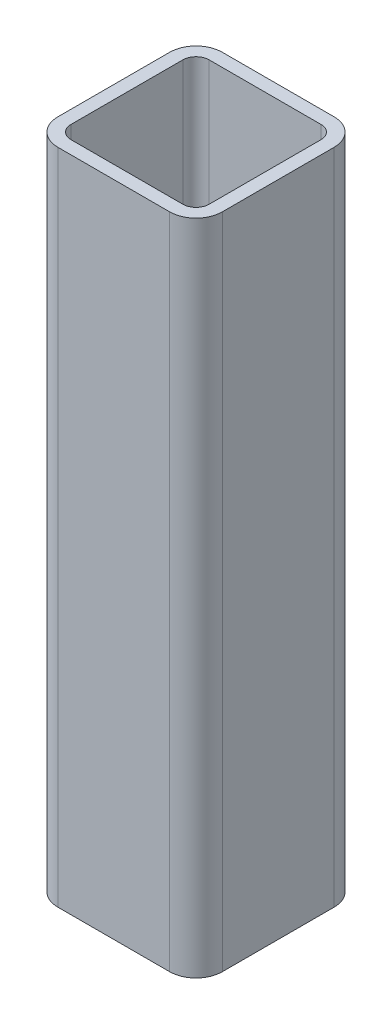
from build123d import *

# Parameters (mm, degrees)
GB_T_6728_2002_SQUARE_HOLLOW_SECTION_STE_DEPTH = 100


with BuildPart() as part:
    # Sketch14 → Gb／t 6728—2002 Square hollow section steel 25×2-example.com(1) (new body)
    with BuildSketch(Plane(origin=(0, 0, 0), x_dir=(-1, 0, 0), z_dir=(0, 1, 0))):
        with BuildLine():
            Line((-8.5, -12.5), (8.5, -12.5))
            ThreePointArc((8.5, -12.5), (11.328427125, -11.328427125), (12.5, -8.5))
            Line((12.5, -8.5), (12.5, 8.5))
            ThreePointArc((12.5, 8.5), (11.328427125, 11.328427125), (8.5, 12.5))
            Line((8.5, 12.5), (-8.5, 12.5))
            ThreePointArc((-8.5, 12.5), (-11.328427125, 11.328427125), (-12.5, 8.5))
            Line((-12.5, 8.5), (-12.5, -8.5))
            ThreePointArc((-12.5, -8.5), (-11.328427125, -11.328427125), (-8.5, -12.5))
        make_face()
        with BuildLine():
            Line((-8.5, -10.5), (8.5, -10.5))
            ThreePointArc((8.5, -10.5), (9.914213562, -9.914213562), (10.5, -8.5))
            Line((10.5, -8.5), (10.5, 8.5))
            ThreePointArc((10.5, 8.5), (9.914213562, 9.914213562), (8.5, 10.5))
            Line((8.5, 10.5), (-8.5, 10.5))
            ThreePointArc((-8.5, 10.5), (-9.914213562, 9.914213562), (-10.5, 8.5))
            Line((-10.5, 8.5), (-10.5, -8.5))
            ThreePointArc((-10.5, -8.5), (-9.914213562, -9.914213562), (-8.5, -10.5))
        make_face(mode=Mode.SUBTRACT)
    extrude(amount=GB_T_6728_2002_SQUARE_HOLLOW_SECTION_STE_DEPTH)


solid = part.part
